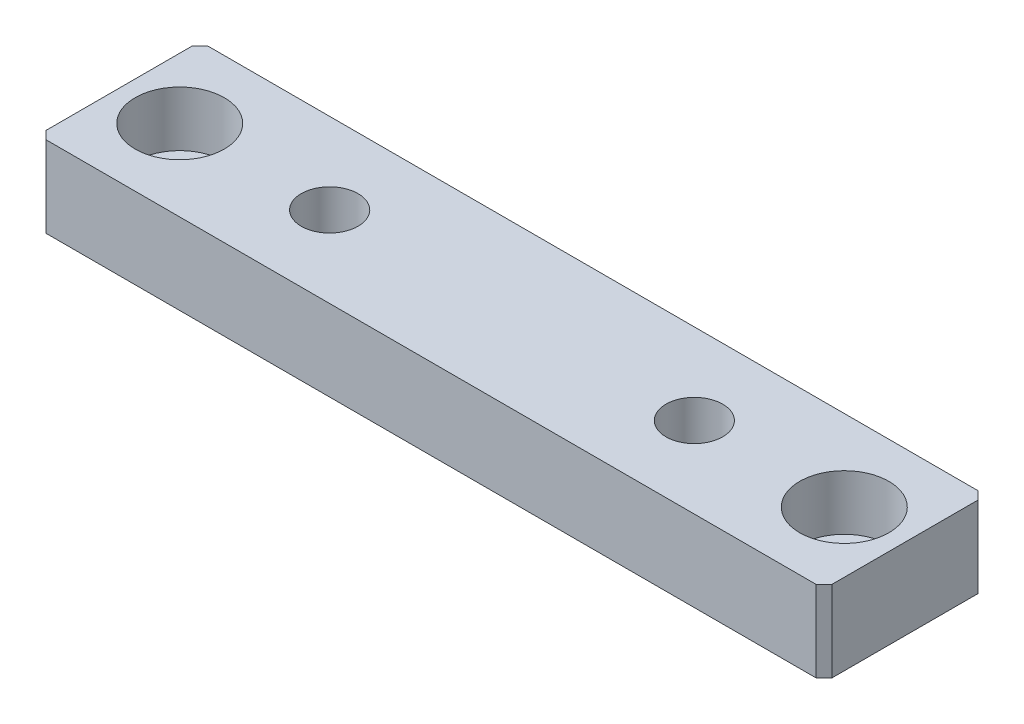
from build123d import *

# Parameters (mm, degrees)
SKETCH_1_W                   = 97
SKETCH_1_H                   = 20
EXTRUDE_1_DEPTH              = 5
M8X1_0_1_D                   = 7
HOLE_WIZARD_M6_1_D           = 6.6
HOLE_WIZARD_M6_1_CBORE_D     = 11
HOLE_WIZARD_M6_1_CBORE_DEPTH = 6.8
CHAMFER_1_SIZE               = 1


with BuildPart() as part:
    # 草图1 → 凸台-拉伸1 (new, symmetric)
    with BuildSketch(Plane(origin=(0, 0, 0), x_dir=(1, 0, 0), z_dir=(0, 1, 0))):
        Rectangle(SKETCH_1_W, SKETCH_1_H)
    extrude(amount=EXTRUDE_1_DEPTH, both=True)

    # M8x1.0 螺纹孔1 (through all)
    with Locations(Plane(origin=(0, 5, 0), x_dir=(1, 0, 0), z_dir=(0, 1, 0))):
        with Locations((-22.5, 0), (22.5, 0)):
            Hole(M8X1_0_1_D / 2)

    # M6 六角圆柱头螺钉的柱形沉头孔1 (through all)
    with Locations(Plane(origin=(0, 5, -3), x_dir=(-1, 0, 0), z_dir=(0, 1, 0))):
        with Locations((41, 3), (-41, 3)):
            CounterBoreHole(HOLE_WIZARD_M6_1_D / 2, HOLE_WIZARD_M6_1_CBORE_D / 2, HOLE_WIZARD_M6_1_CBORE_DEPTH)

    # 倒角1
    chamfer_1_edges = [part.edges().sort_by_distance(p)[0] for p in [
        (48.5, 0, 10),
        (-48.5, 0, 10),
        (-48.5, 0, -10),
        (48.5, 0, -10),
    ]]
    chamfer(chamfer_1_edges, length=CHAMFER_1_SIZE)


solid = part.part
